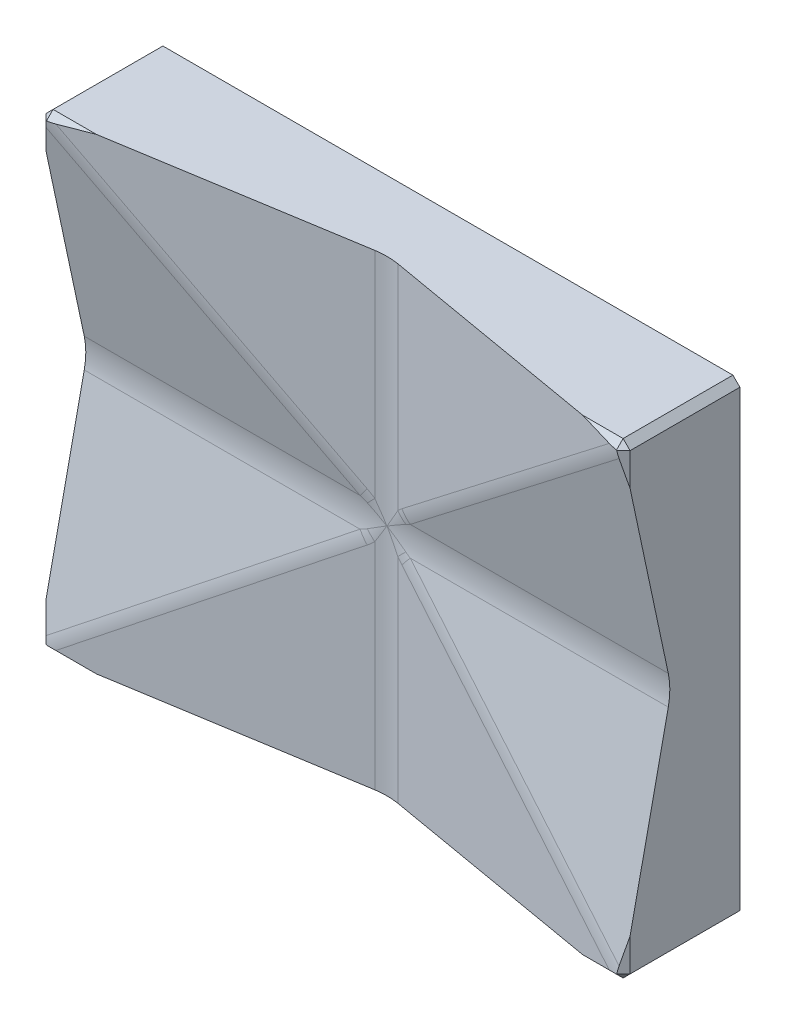
from build123d import *

# Parameters (mm, degrees)
SKETCH1_W           = 25
SKETCH1_H           = 20
BOSS_EXTRUDE1_DEPTH = 5
CHAMFER1_SIZE       = 0.3
CUT_EXTRUDE1_REACH  = 26.109
CUT_EXTRUDE2_DEPTH  = 28.386127875
FILLET1_R           = 2


with BuildPart() as part:
    # Sketch1 → Boss-Extrude1 (new body)
    with BuildSketch(Plane.XY):
        Rectangle(SKETCH1_W, SKETCH1_H)
    extrude(amount=BOSS_EXTRUDE1_DEPTH)

    # Chamfer1
    chamfer1_edges = [part.edges().sort_by_distance(p)[0] for p in [
        (-12.5, 0, 5),
        (0, -10, 5),
        (12.5, 0, 5),
        (12.5, -10, 2.5),
        (-12.5, -10, 2.5),
        (-12.5, 10, 2.5),
        (12.5, 10, 2.5),
        (0, 10, 5),
    ]]
    chamfer(chamfer1_edges, length=CHAMFER1_SIZE)

    # Sketch2 → Cut-Extrude1 (cut, up to next)
    with BuildSketch(Plane(origin=(0, 10, 0), x_dir=(1, 0, 0), z_dir=(0, 1, 0)), mode=Mode.PRIVATE) as cut_extrude1_sk1:
        with BuildLine():
            Line((12.2, -5), (0.90108548, -3.043926058))
            ThreePointArc((0.90108548, -3.043926058), (0.405599363, -3), (-0.090333879, -3.038551394))
            Line((-0.090333879, -3.038551394), (-12.2, -5))
            Line((-12.2, -5), (12.2, -5))
        make_face()
    cut_extrude1_tool1 = extrude(cut_extrude1_sk1.sketch, amount=-CUT_EXTRUDE1_REACH, mode=Mode.PRIVATE) & part.part
    add(cut_extrude1_tool1.solids().sort_by_distance((0.135125, 10, 4.320136))[0], mode=Mode.SUBTRACT)

    # Sketch3 → Cut-Extrude2 (cut, through all)
    with BuildSketch(Plane.ZY.offset(12.5)):
        with BuildLine():
            Line((5, 9.7), (3.065901059, 0.625350625))
            ThreePointArc((3.065901059, 0.625350625), (3, 0), (3.065901059, -0.625350625))
            Line((3.065901059, -0.625350625), (5, -9.7))
            Line((5, -9.7), (5, 9.7))
        make_face()
    extrude(amount=-CUT_EXTRUDE2_DEPTH, mode=Mode.SUBTRACT)

    # Fillet1
    fillet1_edges = [part.edges().sort_by_distance(p)[0] for p in [
        (6.61401009, 5.162675312, 4.032950529),
        (0.963107155, 0.570080363, 3.054663282),
        (0.963107155, -0.570080363, 3.054663282),
        (6.61401009, -5.162675312, 4.032950529),
        (-6.229593142, -5.162675312, 4.032950529),
        (-0.172328062, 0.555254202, 3.051832303),
        (0.373072756, -2e-09, 3),
        (-0.172328062, -0.555254202, 3.051832303),
        (0.405599358, -2e-09, 3),
        (-6.229593142, 5.162675312, 4.032950529),
    ]]
    fillet(fillet1_edges, radius=FILLET1_R)


solid = part.part
